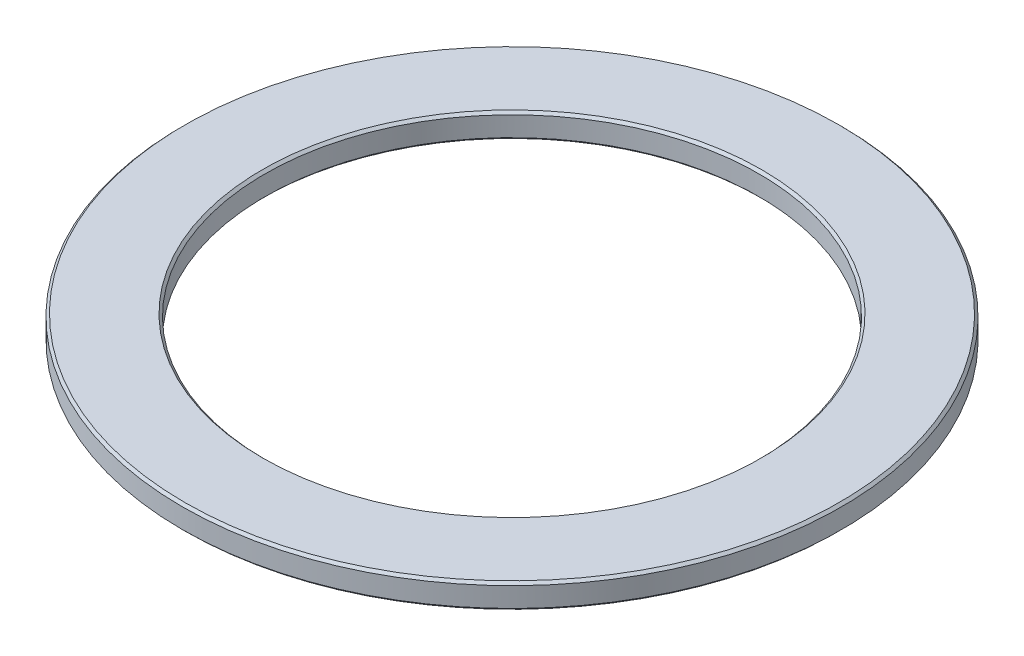
from build123d import *

# Parameters (mm, degrees)
SKETCH1_R           = 40
SKETCH1_R_2         = 30
BOSS_EXTRUDE1_DEPTH = 1.5
CHAMFER1_SIZE       = 0.3


with BuildPart() as part:
    # Sketch1 → Boss-Extrude1 (new, symmetric)
    with BuildSketch(Plane(origin=(0, 0, 0), x_dir=(1, 0, 0), z_dir=(0, 1, 0))):
        with Locations(Location((0, 0, 0), (0, 0, 270))):
            Circle(SKETCH1_R)
        with Locations(Location((0, 0, 0), (0, 0, 270))):
            Circle(SKETCH1_R_2, mode=Mode.SUBTRACT)
    extrude(amount=BOSS_EXTRUDE1_DEPTH, both=True)

    # Chamfer1
    chamfer1_edges = [part.edges().sort_by_distance(p)[0] for p in [
        (0, -1.5, -40),
        (0, 1.5, -40),
        (0, -1.5, -30),
        (0, 1.5, -30),
    ]]
    chamfer(chamfer1_edges, length=CHAMFER1_SIZE)


solid = part.part
